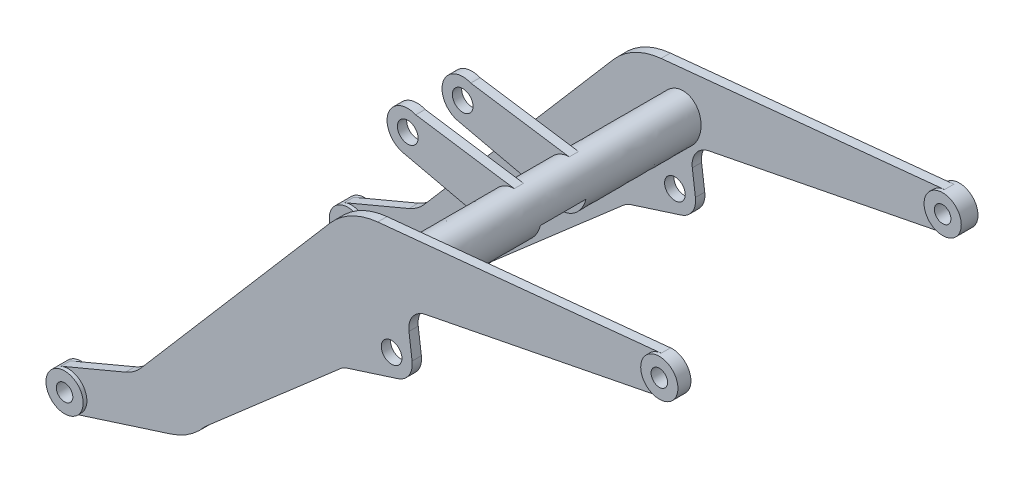
from build123d import *

# Parameters (mm, degrees)
SKETCH_1_9_R        = 40
SKETCH_1_9_R_2      = 50
BOSS_EXTRUDE1_DEPTH = 45
BOSS_EXTRUDE2_START = 18
SKETCH_1_4_R        = 90
SKETCH_1_4_R_2      = 40
BOSS_EXTRUDE2_DEPTH = 18
BOSS_EXTRUDE3_START = 18
SKETCH_1_5_R        = 90
SKETCH_1_5_R_2      = 40
BOSS_EXTRUDE3_DEPTH = 18
SKETCH_1_6_R        = 90
SKETCH_1_6_R_2      = 40
BOSS_EXTRUDE4_DEPTH = 63
SKETCH_1_7_R        = 90
BOSS_EXTRUDE5_DEPTH = 63
SKETCH_1_8_RX       = 125.659756877
SKETCH_1_8_RY       = 99.837004296
BOSS_EXTRUDE6_DEPTH = 663
BOSS_EXTRUDE7_START = 552.5
SKETCH_1_9_2_R      = 100
SKETCH_1_9_2_R_2    = 50
BOSS_EXTRUDE7_DEPTH = 45
SKETCH2_R           = 40
CUT_EXTRUDE1_DEPTH  = 49788.688820018
SKETCH3_R           = 40
CUT_EXTRUDE2_DEPTH  = 49788.688820018
CUT_EXTRUDE3_DEPTH  = 221


with BuildPart() as part:
    # Sketch 1_9 → Boss-Extrude1 (new body)
    with BuildSketch(Plane.XY):
        with BuildLine():
            Line((46764.493197331, 4185.239251674), (46452.152147493, 4053.719390084))
            ThreePointArc((46452.152147493, 4053.719390084), (46402.66618426, 3939.556468955), (46514.523767059, 3885.059548967))
            Line((46514.523767059, 3885.059548967), (46982.465765958, 4034.890698674))
            ThreePointArc((46982.465765958, 4034.890698674), (47073.849116266, 4079.687564008), (47148.481541029, 4148.880605792))
            Line((47148.481541029, 4148.880605792), (47802.541539098, 4718.321446539))
            ThreePointArc((47802.541539098, 4718.321446539), (47819.111250519, 4730.020011667), (47837.700732572, 4738.134376685))
            Line((47837.700732572, 4738.134376685), (48081.909186186, 4816.356275444))
            ThreePointArc((48081.909186186, 4816.356275444), (48135.809793395, 4857.963377024), (48150.576746765, 4924.434148403))
            Line((48150.576746765, 4924.434148403), (48135.440258517, 5041.30699285))
            ThreePointArc((48135.440258517, 5041.30699285), (48153.434870258, 5112.548528391), (48215.258327605, 5152.260271737))
            Line((48215.258327605, 5152.260271737), (49382.281133207, 5382.474576425))
            ThreePointArc((49382.281133207, 5382.474576425), (49453.894200575, 5483.941713279), (49355.973841273, 5560.332907228))
            Line((49355.973841273, 5560.332907228), (47984.319907502, 5424.193649598))
            ThreePointArc((47984.319907502, 5424.193649598), (47857.278403088, 5386.359864507), (47753.417603416, 5303.995591733))
            Line((47753.417603416, 5303.995591733), (46838.575364644, 4239.227151402))
            ThreePointArc((46838.575364644, 4239.227151402), (46804.669066153, 4207.931651), (46764.493197331, 4185.239251674))
        make_face()
        with Locations((46487.079046119, 3970.772951026)):
            Circle(SKETCH_1_9_R, mode=Mode.SUBTRACT)
        with Locations((48051.40501522, 4911.590174628)):
            Circle(SKETCH_1_9_R_2, mode=Mode.SUBTRACT)
    boss_extrude1 = extrude(amount=-BOSS_EXTRUDE1_DEPTH)

    # 草图1<4> → Boss-Extrude2 (add)
    with BuildSketch(Plane.XY.offset(BOSS_EXTRUDE2_START)):
        with Locations((46487.079046119, 3970.772951026)):
            Circle(SKETCH_1_4_R)
        with Locations((46487.079046119, 3970.772951026)):
            Circle(SKETCH_1_4_R_2, mode=Mode.SUBTRACT)
    boss_extrude2 = extrude(amount=-BOSS_EXTRUDE2_DEPTH)

    # 草图1<5> → Boss-Extrude3 (add)
    with BuildSketch(Plane.XY.offset(BOSS_EXTRUDE3_START)):
        with Locations((49364.862836996, 5470.772951026)):
            Circle(SKETCH_1_5_R)
        with Locations((49364.862836996, 5470.772951026)):
            Circle(SKETCH_1_5_R_2, mode=Mode.SUBTRACT)
    extrude(amount=-BOSS_EXTRUDE3_DEPTH)

    # 草图1<6> → Boss-Extrude4 (add)
    with BuildSketch(Plane.XY):
        with Locations((49364.862836996, 5470.772951026)):
            Circle(SKETCH_1_6_R)
        with Locations((49364.862836996, 5470.772951026)):
            Circle(SKETCH_1_6_R_2, mode=Mode.SUBTRACT)
    boss_extrude4 = extrude(amount=-BOSS_EXTRUDE4_DEPTH)

    # 草图1<7> → Boss-Extrude5 (add)
    with BuildSketch(Plane.XY):
        with Locations((46487.079046119, 3970.772951026)):
            Circle(SKETCH_1_7_R)
    boss_extrude5 = extrude(amount=-BOSS_EXTRUDE5_DEPTH)

    # 草图1<8> → Boss-Extrude6 (add)
    with BuildSketch(Plane.XY):
        with Locations(Location((48073.515618599, 5219.948569609), (0, 0, 66.489605314))):
            Ellipse(SKETCH_1_8_RX, SKETCH_1_8_RY)
    boss_extrude6 = extrude(amount=BOSS_EXTRUDE6_DEPTH)

    # Sketch 1_9 2 → Boss-Extrude7 (add)
    # profile 1 of 3: a face of its own
    with BuildSketch(Plane.XY.offset(BOSS_EXTRUDE7_START)):
        with BuildLine():
            Line((47557.654356915, 5222.677683814), (47662.826482923, 5198.558214679))
            Line((47662.826482923, 5198.558214679), (47753.417603416, 5303.995591733))
            ThreePointArc((47753.417603416, 5303.995591733), (47795.418981849, 5345.277345585), (47843.747365572, 5378.932453937))
            Line((47843.747365572, 5378.932453937), (47616.039058549, 5412.871362692))
            ThreePointArc((47616.039058549, 5412.871362692), (47660.433713784, 5376.017854668), (47677.079046119, 5320.772951026))
            ThreePointArc((47677.079046119, 5320.772951026), (47640.551603494, 5243.499187948), (47557.654356915, 5222.677683814))
        make_face()
    # profile 2 of 3: a face of its own
    with BuildSketch(Plane.XY.offset(BOSS_EXTRUDE7_START)):
        with Locations((47577.079046119, 5320.772951026)):
            Circle(SKETCH_1_9_2_R)
        with Locations(Location((47577.079046119, 5320.772951026, 0), (0, 0, 180))):
            Circle(SKETCH_1_9_2_R_2, mode=Mode.SUBTRACT)
    # profile 3 of 3: a face of its own
    with BuildSketch(Plane.XY.offset(BOSS_EXTRUDE7_START)):
        with BuildLine():
            Line((47753.417603416, 5303.995591733), (47662.826482923, 5198.558214679))
            Line((47662.826482923, 5198.558214679), (47998.671509076, 5121.53777162))
            add(Edge.make_bspline(
                [(48092.5354326, 5341.85170086), (47770.125479059, 5347.623127791), (47998.671509076, 5121.53777162)],
                knots=[0.317708152, 0.317708152, 0.317708152, 2.842958608, 2.842958608, 2.842958608], degree=2, weights=[1, 0.303316403, 1]))
            Line((48092.5354326, 5341.85170086), (47843.747365572, 5378.932453937))
            ThreePointArc((47843.747365572, 5378.932453937), (47795.418981849, 5345.277345585), (47753.417603416, 5303.995591733))
        make_face()
    boss_extrude7 = extrude(amount=-BOSS_EXTRUDE7_DEPTH)

    # Mirror1: Boss-Extrude6, Boss-Extrude7 across plane
    add(boss_extrude6.mirror(Plane.XY.offset(663)))
    add(boss_extrude7.mirror(Plane.XY.offset(663)))

    # Mirror2: Boss-Extrude1, Boss-Extrude2, Boss-Extrude4, Boss-Extrude5 across plane
    add(boss_extrude1.mirror(Plane.XY.offset(663)))
    add(boss_extrude2.mirror(Plane.XY.offset(663)))
    add(boss_extrude4.mirror(Plane.XY.offset(663)))
    add(boss_extrude5.mirror(Plane.XY.offset(663)))

    # Sketch2 → Cut-Extrude1 (cut, through all)
    with BuildSketch(Plane.XY.offset(1389)):
        with Locations((49364.862836996, 5470.772951026)):
            Circle(SKETCH2_R)
    extrude(amount=-CUT_EXTRUDE1_DEPTH, mode=Mode.SUBTRACT)

    # Sketch3 → Cut-Extrude2 (cut, through all)
    with BuildSketch(Plane.XY.offset(1389)):
        with Locations((46487.079046119, 3970.772951026)):
            Circle(SKETCH3_R)
    extrude(amount=-CUT_EXTRUDE2_DEPTH, mode=Mode.SUBTRACT)

    # Sketch5 → Cut-Extrude3 (cut)
    with BuildSketch(Plane.XY.offset(552.5)):
        Polygon((47717.278601739, 5369.715122103), (48519.148514072, 5080.278976816), (48183.962905589, 4783.475969073), (47697.072231971, 5313.734277215), align=None)
    extrude(amount=CUT_EXTRUDE3_DEPTH, mode=Mode.SUBTRACT)


solid = part.part
